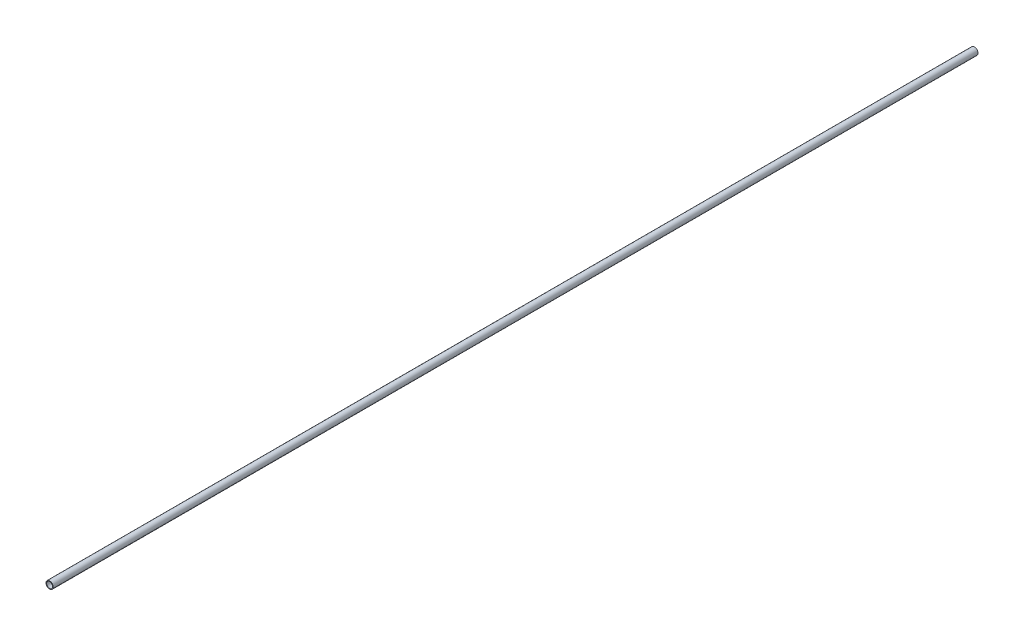
SolidWorks part; units mm, degrees
material "6061-T6 (GB)"
ref_plane "Front Plane" through (0, 0, 0) normal (0, 0, 1) x (1, 0, 0)
ref_plane "Top Plane" through (0, 0, 0) normal (0, 1, 0) x (1, 0, 0)
ref_plane "Right Plane" through (0, 0, 0) normal (1, 0, 0) x (0, 0, -1)
sketch "Sketch1" plane through (0, 0, 0) normal (0, 0, 1) x (1, 0, 0)
  circle A0 centre (0, 0) radius 17.5
  circle A2 centre (0, 0) radius 14.5
  dimension "D1" = 35
  dimension "D2" = 29
extrude "Boss-Extrude1" add sketch "Sketch1" along normal blind 4500
